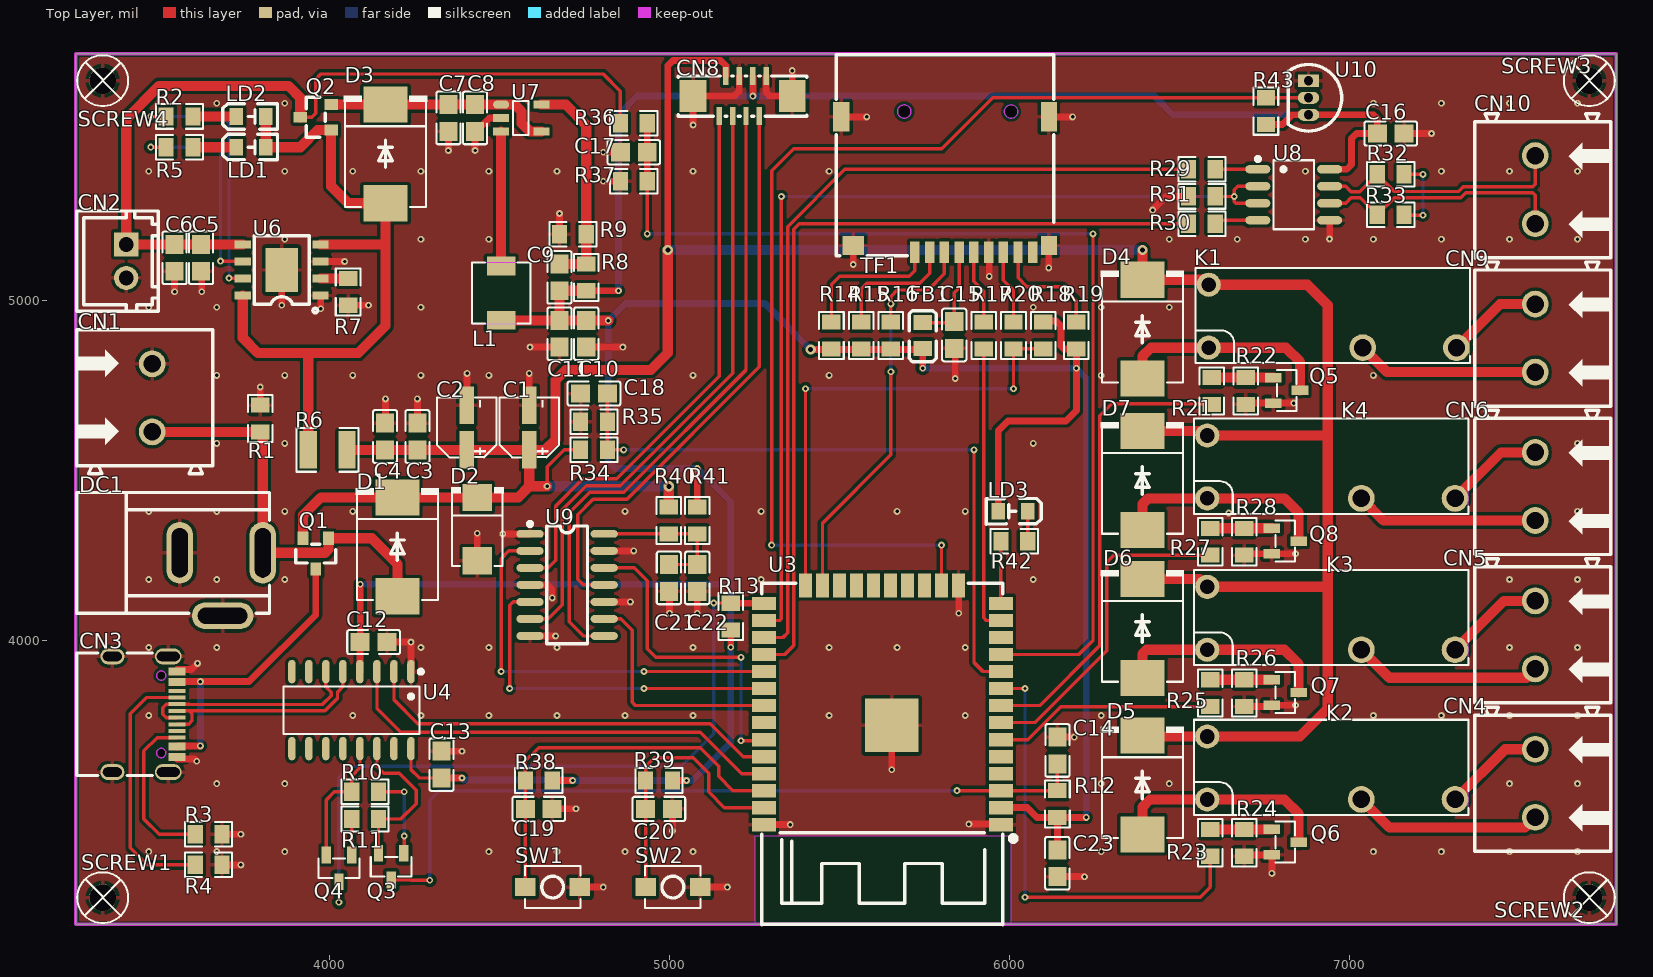
[diagram p0: Top Layer view]
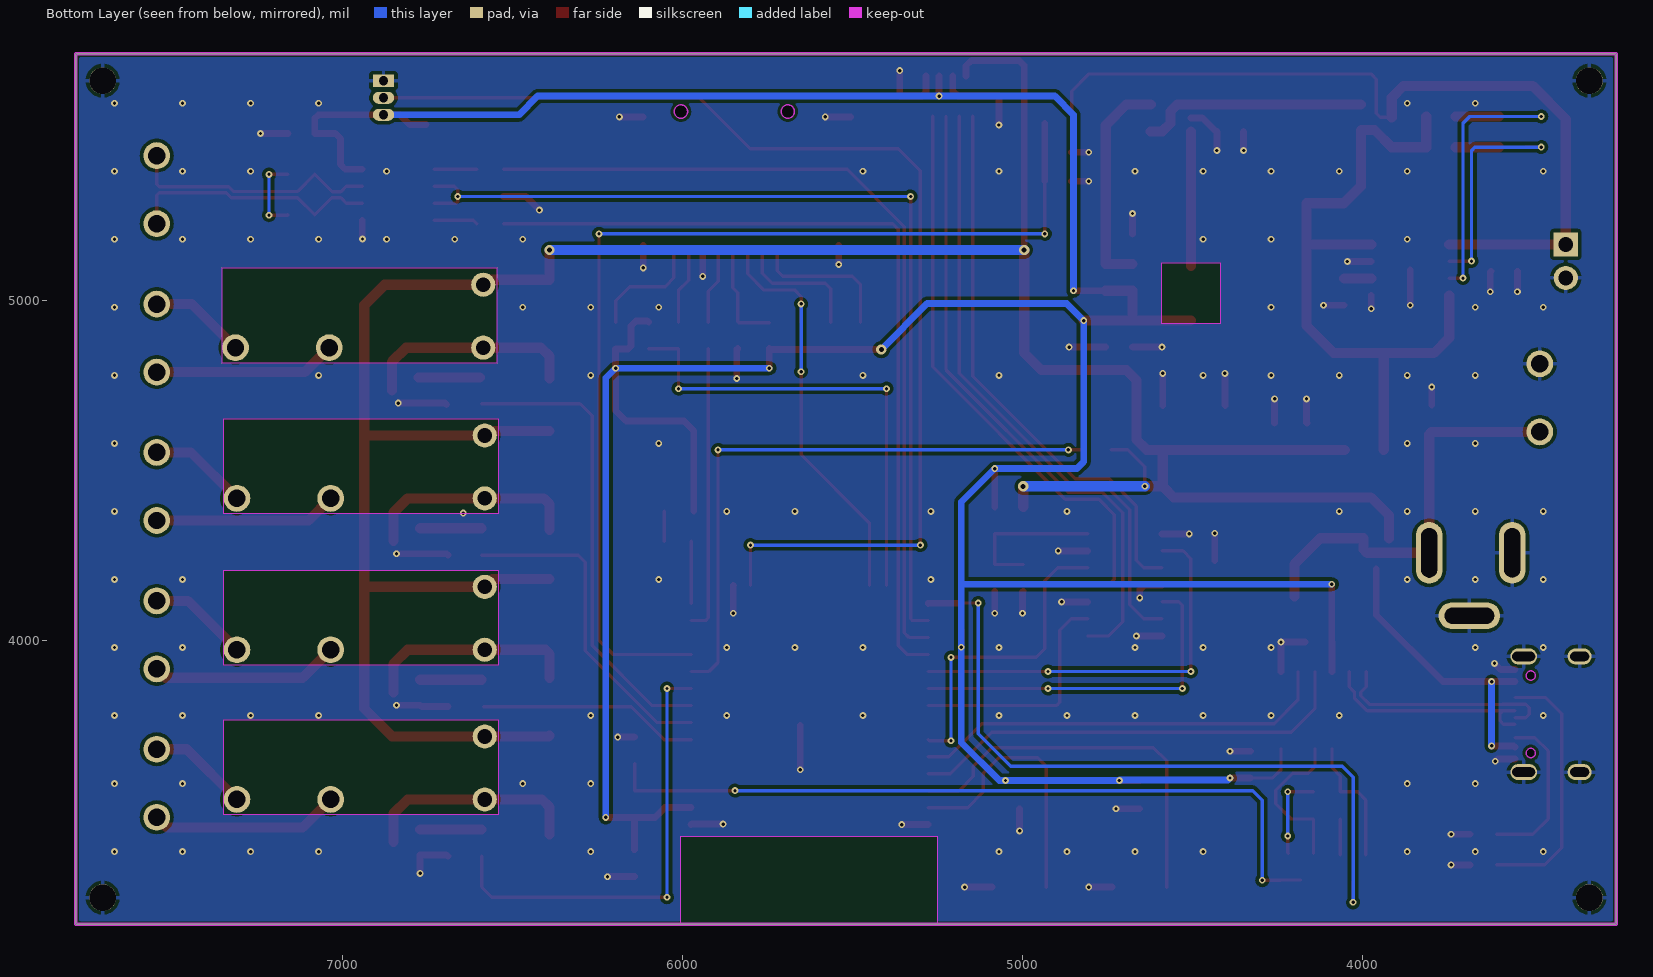
[diagram p1: Bottom Layer view, seen from below]
# Altium PCB MISC49869.pcbdoc
Units mil, origin at the board's own origin, x right, y up, seen from the top; angles counter-clockwise.
Board outline 4527.56 x 2559.06 mil, 2 copper layers (Top Layer, Bottom Layer), stack 62.206 mil thick; 114 components, 80 nets, 367 pads, 217 vias.

## Layer stack, top to bottom
Top Solder Mask Layer: solder mask 0.394, Dk 3.3
Top Layer: signal copper 1.379
Dielectric1: surface 59.449, FR4, Dk 4.5
Bottom Layer: signal copper 1.378
Bottom Solder Mask Layer: solder mask 0.394, Dk 3.3

## Board outline
3255,3165 7782.56,3165 7782.56,5724.06 3255,5724.06

## Design rules (kind name [scope] priority, off if disabled: settings)
BoardOutlineClearance copperThickness2oz_1 [All] p2 off: genericclearance=7.99 ignorepadtopadclearanceinfootprint=FALSE except(0: Arc-SplitContinuation Track-SplitContinuation SMDPad-SplitContinuation THPad-SplitContinuation Via-SplitContinuation Fill-SplitContinuation Region-SplitContinuation Poly-SplitContinuation Text-SplitContinuation Hole-SplitContinuation; 5.98: Arc-CutoutEdge Track-CutoutEdge SMDPad-CutoutEdge THPad-CutoutEdge Via-CutoutEdge Text-CutoutEdge; 6.89: Hole-OutlineEdge Hole-CutoutEdge; 10: Poly-OutlineEdge Poly-CutoutEdge; 11.81: Arc-OutlineEdge Track-OutlineEdge SMDPad-OutlineEdge THPad-OutlineEdge Via-OutlineEdge Fill-OutlineEdge Region-OutlineEdge Text-OutlineEdge Fill-CutoutEdge Region-CutoutEdge)
BoardOutlineClearance Plane_innerPlane_1 [All] p4 off: genericclearance=8 ignorepadtopadclearanceinfootprint=FALSE except(0: Arc-SplitContinuation Track-SplitContinuation SMDPad-SplitContinuation THPad-SplitContinuation Via-SplitContinuation Fill-SplitContinuation Region-SplitContinuation Poly-SplitContinuation Text-SplitContinuation Hole-SplitContinuation; 7: SMDPad-CutoutEdge THPad-CutoutEdge; 8: Arc-OutlineEdge Track-OutlineEdge SMDPad-OutlineEdge THPad-OutlineEdge Via-OutlineEdge Fill-OutlineEdge Region-OutlineEdge Text-OutlineEdge Hole-OutlineEdge Arc-CutoutEdge Track-CutoutEdge Via-CutoutEdge Fill-CutoutEdge Region-CutoutEdge Text-CutoutEdge Hole-CutoutEdge; 10: Poly-OutlineEdge Poly-CutoutEdge)
BoardOutlineClearance Copper_copperRegion_1 [All] p6 off: genericclearance=8 ignorepadtopadclearanceinfootprint=FALSE except(0: Arc-SplitContinuation Track-SplitContinuation SMDPad-SplitContinuation THPad-SplitContinuation Via-SplitContinuation Fill-SplitContinuation Region-SplitContinuation Poly-SplitContinuation Text-SplitContinuation Hole-SplitContinuation; 7: SMDPad-CutoutEdge THPad-CutoutEdge; 8: Arc-OutlineEdge Track-OutlineEdge SMDPad-OutlineEdge THPad-OutlineEdge Via-OutlineEdge Fill-OutlineEdge Region-OutlineEdge Text-OutlineEdge Hole-OutlineEdge Arc-CutoutEdge Track-CutoutEdge Via-CutoutEdge Fill-CutoutEdge Region-CutoutEdge Text-CutoutEdge Hole-CutoutEdge; 10: Poly-OutlineEdge Poly-CutoutEdge)
BoardOutlineClearance copperThickness1oz_1 [All] p8: genericclearance=8 ignorepadtopadclearanceinfootprint=FALSE except(0: Arc-SplitContinuation Track-SplitContinuation SMDPad-SplitContinuation THPad-SplitContinuation Via-SplitContinuation Fill-SplitContinuation Region-SplitContinuation Poly-SplitContinuation Text-SplitContinuation Hole-SplitContinuation; 7: SMDPad-CutoutEdge THPad-CutoutEdge; 8: Arc-OutlineEdge Track-OutlineEdge SMDPad-OutlineEdge THPad-OutlineEdge Via-OutlineEdge Fill-OutlineEdge Region-OutlineEdge Text-OutlineEdge Hole-OutlineEdge Arc-CutoutEdge Track-CutoutEdge Via-CutoutEdge Fill-CutoutEdge Region-CutoutEdge Text-CutoutEdge Hole-CutoutEdge; 10: Poly-OutlineEdge Poly-CutoutEdge)
Clearance copperThickness2oz [All] p1 off: gap=7.99 ignorepadtopadclearanceinfootprint=FALSE except(5.98: SMDPad-Track SMDPad-SMDPad THPad-Track SMDPad-THPad THPad-THPad Track-Via SMDPad-Via THPad-Via Via-Via Fill-SMDPad Region-SMDPad Fill-THPad Region-THPad Fill-Via Region-Via Fill-Fill Fill-Region Region-Region Arc-Track Arc-SMDPad Arc-THPad Arc-Via Fill-Arc Region-Arc Arc-Arc Text-Track SMDPad-Text Text-THPad Text-Via Fill-Text Region-Text Arc-Text Text-Text; 6.89: Hole-Track Hole-SMDPad Hole-THPad Hole-Via Fill-Hole Region-Hole Hole-Arc Hole-Text; 10: Poly-Track Poly-SMDPad Poly-THPad Poly-Via Poly-Fill Poly-Region Poly-Poly Poly-Arc Poly-Text Poly-Hole; 11.81: Fill-Track Region-Track)
Clearance Plane_innerPlane [All] p3 off: gap=8 ignorepadtopadclearanceinfootprint=FALSE except(7: SMDPad-SMDPad SMDPad-THPad THPad-THPad; 10: Poly-Track Poly-SMDPad Poly-THPad Poly-Via Poly-Fill Poly-Region Poly-Poly Poly-Arc Poly-Text Poly-Hole)
Clearance Copper_copperRegion [All] p5 off: gap=8 ignorepadtopadclearanceinfootprint=FALSE except(7: SMDPad-SMDPad SMDPad-THPad THPad-THPad; 10: Poly-Track Poly-SMDPad Poly-THPad Poly-Via Poly-Fill Poly-Region Poly-Poly Poly-Arc Poly-Text Poly-Hole)
Clearance copperThickness1oz [All] p7: gap=8 ignorepadtopadclearanceinfootprint=FALSE except(7: SMDPad-SMDPad SMDPad-THPad THPad-THPad; 10: Poly-Track Poly-SMDPad Poly-THPad Poly-Via Poly-Fill Poly-Region Poly-Poly Poly-Arc Poly-Text Poly-Hole)
DiffPairsRouting differentialPair [All] p1: maxlimit=8 minlimit=8 mostfreqgap=8 toplayer_minwidth=10 toplayer_prefwidth=10 toplayer_maxwidth=100 toplayer_mingap=8 toplayer_prefgap=8 toplayer_maxgap=8 bottomlayer_minwidth=10 bottomlayer_prefwidth=10 bottomlayer_maxwidth=100 bottomlayer_mingap=8 bottomlayer_prefgap=8 bottomlayer_maxgap=8 maxuncoupledlength=8
HoleToHoleClearance otherClearance [All] p1: gap=11.81 allowstackedmicrovias=TRUE
Length netLength [All] p1: minlimit=0 maxlimit=0
PasteMaskExpansion pasteMaskExpansion [All] p1: expansion=0
PlaneConnect innerPlane [All] p1: planeconnectstyle=Relief reliefexpansion=20 reliefentries=4 reliefconductorwidth=10 reliefairgap=10
PolygonConnect copperRegion [All] p1: connectstyle=Relief reliefconductorwidth=10 reliefentries=4 polygonreliefangle="90 Angle" airgapwidth=10 via.connectstyle=Relief via.reliefconductorwidth=10 via.reliefentries=4 via.polygonreliefangle="90 Angle" via.airgapwidth=10
RoutingVias viaSize [All] p1: holewidth=10 width=20 viastyle="Through Hole" minholewidth=10 minwidth=20 maxholewidth=248.03 maxwidth=393.7
SolderMaskExpansion solderMaskExpansion [IsVia] p1: expansion=-1000 istentingtop=TRUE
SolderMaskExpansion solderMaskExpansion [All] p2: expansion=2.01 istentingtop=FALSE
Width copperThickness2oz_2 [All] p1 off: maxlimit=100 minlimit=8 preferedwidth=10
Width copperThickness1oz_2 [All] p2: maxlimit=100 minlimit=8 preferedwidth=8

## Components (designator, comment, footprint, x,y, rotation, side; value= is the part's Value field where it differs from the comment)
C1 "47uF" C_Ele_SMD_4x5.5mm 4587.93,4620.75 r90 top
C2 "47uF" C_Ele_SMD_4x5.5mm 4403.8,4620.75 r90 top
C3 "100nF" C0805 4258.8,4599.37 r270 top
C4 "10nF" C0805 4163.8,4599.37 r270 top
C5 "10uF" C0805 3622.97,5124.54 r90 top
C6 "10nF" C0805 3545,5124.54 r90 top
C7 "10uF" C0805 4349.92,5535.76 r90 top
C8 "10uF" C0805 4428.44,5535.76 r90 top
C9 "NF" C0805 4676.48,5067.13 r90 top
C10 "22uF" C0805 4755.22,4901.43 r90 top
C11 "22uF" C0805 4676.48,4901.43 r90 top
C12 "100nF" C0805 4130,3995 r0 top
C13 "100nF" C0805 4330,3635 r270 top
C14 "1uF" C0805 6140.35,3676.45 r90 top
C15 "10uF" C0805 5836.91,4897.76 r270 top
C16 "100nF" C0805 7120,5490 r0 top
C17 "100nF" C0805 4895,5435 r180 top
C18 "100nF" C0805 4777.97,4725.53 r180 top
C19 "100nF" C0805 4615.7,3504.84 r180 top
C20 "100nF" C0805 4968.94,3504.84 r180 top
C21 "100nF" C0805 4997.99,4183.61 r90 top
C22 "10nF" C0805 5081.52,4183.61 r90 top
C23 "100nF" C0805 6140,3345 r270 top
CN1 "" CONN-TH_2P-P5.00_WJ500V-5.08-2P 3479.21,4712.95 r90 top
CN2 "" CONN-TH_2P-P2.50_HX25003-2A 3402.83,5114.7 r270 top
CN3 "" USB_TYPE-C-16P 3457.17,3787.83 r270 top
CN4 "" CONN-TH_2P-P5.00_WJ500V-5.08-2P 7545,3580 r270 top locked
CN5 "" CONN-TH_2P-P5.00_WJ500V-5.08-2P 7545,4016.2 r270 top locked
CN6 "" CONN-TH_2P-P5.00_WJ500V-5.08-2P 7545,4452.5 r270 top locked
CN8 "" FPC-SMD_8P-P0.50_AFC11-S08ICC-00 5215,5600 r0 top
CN9 "" CONN-TH_2P-P5.00_WJ500V-5.08-2P 7545,4888.7 r270 top locked
CN10 "" CONN-TH_2P-P5.00_WJ500V-5.08-2P 7545,5325 r270 top locked
D1 "" SMC_L6.9-W5.9-LS7.9-RD 4200,4275 r270 top
D2 "" SMB_L4.6-W3.6-LS5.3-RD 4435,4327.19 r270 top
D3 "" SMC_L6.9-W5.9-LS7.9-RD 4165,5430 r270 top
D4 "" SMC_L6.9-W5.9-LS7.9-RD 6390,4915 r270 top
D5 "" SMC_L6.9-W5.9-LS7.9-RD 6390,3575 r270 top
D6 "" SMC_L6.9-W5.9-LS7.9-RD 6390,4035 r270 top
D7 "" SMC_L6.9-W5.9-LS7.9-RD 6390,4470 r270 top
DC1 "" DC-005_2.5 3677.36,4245 r180 top
FB1 "10uH" L0805 5744.14,4896.17 r90 top
K1 "" RELAY-TH_G5NB-1A-E-DCXX 6949.3,4953.03 r0 top
K2 "" RELAY-TH_G5NB-1A-E-DCXX 6945,3625 r0 top
K3 "" RELAY-TH_G5NB-1A-E-DCXX 6945,4065 r0 top
K4 "" RELAY-TH_G5NB-1A-E-DCXX 6945,4510 r0 top
L1 "2.2uH" IND-SMD_L4.4-W4.2 4505,5020.64 r90 top
LD1 "" LED_0805 3771.66,5449.74 r0 top
LD2 "" LED_0805 3771.66,5539.92 r0 top
LD3 "" LED_0805 6007.53,4380 r180 top
Q1 "" SOT-23_L2.9-W1.3-P1.90-LS2.4-BR 3960,4255 r90 top
Q2 "" SOT-23_L2.9-W1.3-P1.90-LS2.4-BR 3960,5537.73 r0 top
Q3 "" SOT-23-3_L2.9-W1.3-P1.90-LS2.4-BR 4181.77,3335 r90 top
Q4 "" SOT-23-3_L2.9-W1.3-P1.90-LS2.4-BR 4028.23,3330 r90 top
Q5 "" SOT-23-3_L2.9-W1.3-P1.90-LS2.4-BR 6814.3,4735 r180 top
Q6 "" SOT-23-3_L2.9-W1.3-P1.90-LS2.4-BR 6810,3406.97 r180 top
Q7 "" SOT-23-3_L2.9-W1.3-P1.90-LS2.4-BR 6810,3846.97 r180 top
Q8 "" SOT-23-3_L2.9-W1.3-P1.90-LS2.4-BR 6810,4291.97 r180 top
R1 "10K" R0805 3797.04,4652.32 r270 top
R2 "1.5K" R0805 3559.69,5540.12 r0 top
R3 "5.1K" R0805 3645,3430 r180 top
R4 "5.1K" R0805 3645,3340 r180 top
R5 "1.5K" R0805 3559.69,5449.94 r0 top
R6 "100mΩ" R1210 3995,4560 r180 top
R7 "1.5K" R0805 4055,5024.54 r270 top
R8 "180K" R0805 4755.22,5067.13 r270 top
R9 "40K" R0805 4715.85,5194.4 r0 top
R10 "1K" R0805 4105,3555 r180 top
R11 "1K" R0805 4105,3475 r0 top
R12 "10K" R0805 6140.35,3519.14 r270 top
R13 "10K" R0805 5180,4070 r270 top
R14 "2.2K" R0805 5476.02,4896.17 r270 top
R15 "2.2K" R0805 5563.43,4896.17 r270 top
R16 "10K" R0805 5650.84,4896.17 r270 top
R17 "10R" R0805 5923.79,4896.17 r270 top
R18 "2.2K" R0805 6098.61,4896.17 r90 top
R19 "2.2K" R0805 6196.02,4896.17 r270 top
R20 "220R" R0805 6011.2,4896.17 r270 top
R21 "4.7K" R0805 6594.3,4733.03 r270 top
R22 "4.7K" R0805 6693.38,4733.03 r90 top
R23 "4.7K" R0805 6590,3405 r270 top
R24 "4.7K" R0805 6689.08,3405 r90 top
R25 "4.7K" R0805 6590,3845 r270 top
R26 "4.7K" R0805 6689.08,3845 r90 top
R27 "4.7K" R0805 6590,4290 r270 top
R28 "4.7K" R0805 6689.08,4290 r90 top
R29 "300R" R0805 6565,5385 r180 top
R30 "300R" R0805 6565,5225 r180 top
R31 "10K" R0805 6565,5305 r180 top
R32 "120R" R0805 7120,5370 r0 top
R33 "0R" R0805 7120,5250.89 r0 top
R34 "100K" R0805 4777.97,4560 r0 top
R35 "100K" R0805 4777.97,4643.03 r180 top
R36 "100K" R0805 4895,5520 r180 top
R37 "100K" R0805 4895,5350 r0 top
R38 "10K" R0805 4615.7,3588.13 r0 top
R39 "10K" R0805 4968.94,3588.13 r0 top
R40 "0R" R0805 4997.99,4352.42 r90 top
R41 "0R" R0805 5081.52,4352.42 r90 top
R42 "1.5K" R0805 6013.44,4291.81 r180 top
R43 "4.7K" R0805 6753.35,5555.7 r270 top
SCREW1 "" M2螺丝 3333.7,3243.7 r0 top locked
SCREW2 "" M2螺丝 7703.8,3243.7 r0 top locked
SCREW3 "" M2螺丝 7703.8,5645.3 r0 top locked
SCREW4 "" M2螺丝 3333.7,5645.3 r0 top locked
SW1 "" Key_SMD_3x4x2 4656.45,3274.84 r0 top
SW2 "" Key_SMD_3x4x2 5009.69,3274.84 r0 top
TF1 "" TF-SMD_TF-CARD-H1.8 5810,5340 r180 top
U3 "" WIFIM-SMD_ESP-WROOM-32 5625.62,3810.1 r180 top
U4 "" SOP-16_L10.0-W3.9-P1.27-LS6.0-BL 4065,3795 r180 top
U6 "" ESOP-8_L4.9-W3.9-P1.27-LS6.0-BL-EP 3860.04,5088.91 r90 top
U7 "" SOT_XDC 4505,5575.13 r0 top
U8 "" SOP-8_L4.9-W3.9-P1.27-LS6.0-BL 6835,5310 r270 top
U9 "" SOIC-14_L8.6-W3.8-P1.27-LS6.0-BL 4698.91,4163.05 r270 top
U10 "" TO-92-3_L4.9-W3.7-P1.27-L 6878.35,5595.07 r270 top

## Footprints (in the part's own frame and the unit in brackets; to place one, negate y for a bottom-side part, rotate by r counter-clockwise, add the part's x,y. Pads: shape width x height; smd on the part's side, far side on the other; paste and mask are expansions set on the pad)
C0805 [mm]
  rect 1.41x1.35 smd paste-100 mask+0.051: 1(-1,0) 2(1,0)
  silkscreen extent -1.96,-0.9 1.96,0.9
C_Ele_SMD_4x5.5mm [mm]
  rect 2.8x1.1 smd paste+0 mask+0.051: 1(-1.543,0) 2(1.778,0)
  silkscreen extent -2.1,-2.23 2.35,2.23
CONN-TH_2P-P2.50_HX25003-2A [mm]
  rect 1.8x1.8 hole 1.1 paste+0 mask+0.05: 1(-1.25,0)
  round 1.8 hole 1.1 paste+0 mask+0.05: 2(1.25,0)
  silkscreen extent -3.75,-3.7 3.75,2.41
CONN-TH_2P-P5.00_WJ500V-5.08-2P [mm]
  round 2 hole 1.3: 1(-2.54,0) 2(2.54,0)
  silkscreen extent -5.68,-4.52 5.08,5.64
DC-005_2.5 [mm]
  oval 2x4.6 hole 1.2 slot 3.7 at 90 deg paste+0 mask+0.051: 1(-3.227,-0.318) 2(2.973,-0.318)
  oval 4.6x2 hole 1.2 slot 3.7 at 0 deg paste+0 mask+0.051: 3(-0.227,4.382)
  silkscreen extent -3.73,-4.82 10.67,4.18
ESOP-8_L4.9-W3.9-P1.27-LS6.0-BL-EP [mm]
  rect 0.6x1.2 smd: 1(-1.905,-2.908) 2(-0.635,-2.908) 3(0.635,-2.908) 4(1.905,-2.908) 5(1.905,2.908) 6(0.635,2.908) 7(-0.635,2.908) 8(-1.905,2.908)
  rect 3.3x2.4 smd: 9(0,0)
  silkscreen extent -3.2,-2.67 2.55,2.05
FPC-SMD_8P-P0.50_AFC11-S08ICC-00 [mm]
  rect 0.4x1.35 smd: 1(-1.75,-1.5) 2(-1.25,1.5) 3(-0.75,-1.5) 4(-0.25,1.5) 5(0.25,-1.5) 6(0.75,1.5) 7(1.25,-1.5) 8(1.75,1.5)
  rect 2x2.4 smd: 9(3.7,0) 10(-3.7,0)
  silkscreen extent -4.81,-1.5 4.8,1.5
IND-SMD_L4.4-W4.2 [mm]
  rect 1.4x2.12 smd: 1(2.028,0) 2(-2.028,0)
  silkscreen extent -2.28,-2.18 2.28,2.18
Key_SMD_3x4x2 [mm]
  rect 1.53x1.36 smd paste+0 mask+0.051: 1(-2.035,0) 2(2.035,0)
  silkscreen extent -2.08,-1.58 2.08,1.58
L0805 [mil]
  rect 44.59x54.21 smd paste-3937.01 mask+2: 1(-38.04,0) 2(38.04,0)
  silkscreen extent -77,-40 73,40
LED_0805 [mm]
  rect 1x1.25 smd paste+0 mask+0.051: 1(-1.15,0.005) 2(1.05,0.005)
  silkscreen extent -2.15,-0.94 1.93,0.97
M2螺丝 [mm]
  round 2 hole 2: 1(0,0)
  silkscreen extent -1.9,-1.9 1.9,1.9
R0805 [mm]
  rect 1.133x1.377 smd paste-100 mask+0.051: 1(-1,0) 2(1,0)
  silkscreen extent -1.76,-0.92 1.76,0.92
R1210 [mil]
  rect 50.49x110.55 smd paste-3937.01 mask+2: 1(-56.74,0) 2(56.74,0)
  silkscreen extent -91,-64 91,64
RELAY-TH_G5NB-1A-E-DCXX [mm]
  round 1.8 hole 1.1: 1(-9.25,-2.35) 4(-9.25,2.35)
  round 2 hole 1.3: 2(2.25,-2.35) 3(9.25,-2.35)
  silkscreen extent -10.25,-3.5 10.25,3.6
SMB_L4.6-W3.6-LS5.3-RD [mil]
  rect 80.61x86.31 smd: 1(-92.94,0) 2(92.94,0)
  silkscreen extent -123,-77 108,77
SMC_L6.9-W5.9-LS7.9-RD [mm]
  rect 2.7x3.3 smd: 1(-3.686,0) 2(3.686,0)
  silkscreen extent -4.36,-3.1 3.98,3.1
SOIC-14_L8.6-W3.8-P1.27-LS6.0-BL [mil]
  oval 22.6x80.24 smd: 1(-150,-109.02) 2(-100,-109.02) 3(-50,-109.02) 4(0,-109.02) 5(50,-109.02) 6(100,-109.02) 7(150,-109.02) 8(150,109.02) 9(100,109.02) 10(50,109.02) 11(0,109.02) 12(-50,109.02) 13(-100,109.02) 14(-150,109.02)
  silkscreen extent -185,-115 173,60
SOP-8_L4.9-W3.9-P1.27-LS6.0-BL [mm]
  oval 0.63x1.865 smd: 1(-1.905,-2.682) 2(-0.635,-2.682) 3(0.635,-2.682) 4(1.905,-2.682) 5(1.905,2.682) 6(0.635,2.682) 7(-0.635,2.682) 8(-1.905,2.682)
  silkscreen extent -2.82,-2.83 2.58,1.52
SOP-16_L10.0-W3.9-P1.27-LS6.0-BL [mm]
  oval 0.56x1.745 smd: 1(-4.445,-2.872) 2(-3.175,-2.872) 3(-1.905,-2.872) 4(-0.635,-2.872) 5(0.635,-2.872) 6(1.905,-2.872) 7(3.175,-2.872) 8(4.445,-2.872) 9(4.445,2.872) 10(3.175,2.872) 11(1.905,2.872) 12(0.635,2.872) 13(-0.635,2.872) 14(-1.905,2.872) 15(-3.175,2.872) 16(-4.445,2.872)
  silkscreen extent -5.33,-3.02 5.08,1.77
SOT-23-3_L2.9-W1.3-P1.90-LS2.4-BR [mm]
  rect 1.25x0.7 smd: 1(1,-0.95) 2(1,0.95) 3(-1,0)
  silkscreen extent -0.73,-1.53 0.73,1.53
SOT-23_L2.9-W1.3-P1.90-LS2.4-BR [mm]
  rect 1x0.8 smd: 1(1.15,-0.95) 2(1.15,0.95) 3(-1.15,0)
  silkscreen extent -0.7,-1.5 0.7,1.5
SOT_XDC [mm]
  oval 1.2x0.6 smd: 1(0,0)
  rect 1.2x0.6 smd: 2(0,-1) 3(0,-2) 4(3,-2) 5(3,0)
  silkscreen extent 0.89,-2.29 2.03,0.25
TF-SMD_TF-CARD-H1.8 [mm]
  rect 0.7x1.6 smd paste+0 mask+0.05: 1(2.25,5.05) 2(1.15,5.05) 3(0.05,5.05) 4(-1.05,5.05) 5(-2.15,5.05) 6(-3.25,5.05) 7(-4.35,5.05) 8(-5.45,5.05) 9(-6.55,5.05)
  rect 1.2x1.4 smd paste+0 mask+0.05: 10(-7.747,4.55)
  rect 1.2x2.2 smd paste+0 mask+0.05: 11(-7.75,-5.05) 12(7.75,-5.05)
  rect 1.6x1.4 smd paste+0 mask+0.05: 13(6.85,4.55)
  Board Outline Layer circle w0.003: c3.05,-5.45 r0.5
  Board Outline Layer circle w0.003: c-4.93,-5.45 r0.5
  Board Outline Layer region: 2.55,-5.45 2.6,-5.233 2.738,-5.059 2.939,-4.962 3.161,-4.962 3.362,-5.059 3.501,-5.233 3.55,-5.45 3.55,-5.45 3.501,-5.667 3.362,-5.841 3.161,-5.937 2.939,-5.937 2.738,-5.841 2.6,-5.667 2.55,-5.45
  Board Outline Layer region: 2.55,-5.45 2.56,-5.352 2.588,-5.259 2.634,-5.172 2.696,-5.096 2.772,-5.034 2.859,-4.988 2.952,-4.96 3.05,-4.95 3.148,-4.96 3.241,-4.988 3.328,-5.034 3.404,-5.096 3.466,-5.172 3.512,-5.259 3.54,-5.352 3.55,-5.45 3.54,-5.547 3.512,-5.641 3.466,-5.728 3.404,-5.804 3.328,-5.866 3.241,-5.912 3.148,-5.94 3.05,-5.95 2.952,-5.94 2.859,-5.912 2.772,-5.866 2.696,-5.804 2.634,-5.728 2.588,-5.641 2.56,-5.547
  Board Outline Layer region: -5.43,-5.45 -5.381,-5.233 -5.242,-5.059 -5.041,-4.962 -4.819,-4.962 -4.618,-5.059 -4.48,-5.233 -4.43,-5.45 -4.43,-5.45 -4.48,-5.667 -4.618,-5.841 -4.819,-5.937 -5.041,-5.937 -5.242,-5.841 -5.381,-5.667 -5.43,-5.45
  Board Outline Layer region: -5.43,-5.45 -5.421,-5.352 -5.392,-5.259 -5.346,-5.172 -5.284,-5.096 -5.208,-5.034 -5.121,-4.988 -5.028,-4.96 -4.93,-4.95 -4.833,-4.96 -4.739,-4.988 -4.652,-5.034 -4.577,-5.096 -4.514,-5.172 -4.468,-5.259 -4.44,-5.352 -4.43,-5.45 -4.44,-5.547 -4.468,-5.641 -4.514,-5.728 -4.577,-5.804 -4.652,-5.866 -4.739,-5.912 -4.833,-5.94 -4.93,-5.95 -5.028,-5.94 -5.121,-5.912 -5.208,-5.866 -5.284,-5.804 -5.346,-5.728 -5.392,-5.641 -5.421,-5.547
  Multi-Layer board cut-out: 2.55,-5.45 2.6,-5.233 2.738,-5.059 2.939,-4.962 3.161,-4.962 3.362,-5.059 3.501,-5.233 3.55,-5.45 3.55,-5.45 3.501,-5.667 3.362,-5.841 3.161,-5.937 2.939,-5.937 2.738,-5.841 2.6,-5.667 2.55,-5.45
  Multi-Layer board cut-out: -5.43,-5.45 -5.381,-5.233 -5.242,-5.059 -5.041,-4.962 -4.819,-4.962 -4.618,-5.059 -4.48,-5.233 -4.43,-5.45 -4.43,-5.45 -4.48,-5.667 -4.618,-5.841 -4.819,-5.937 -5.041,-5.937 -5.242,-5.841 -5.381,-5.667 -5.43,-5.45
  silkscreen extent -8.13,-9.68 8.13,5.3
TO-92-3_L4.9-W3.7-P1.27-L [mm]
  rect 0.9x1.6 hole 0.7 paste+0 mask+0.051: 1(-1.27,0)
  oval 0.9x1.6 hole 0.7 paste+0 mask+0.051: 2(0,0) 3(1.27,0)
  silkscreen extent -2.48,-1.5 2.48,2.48
USB_TYPE-C-16P [mm]
  oval 1.2x2 hole 0.7 slot 1.7 at 90 deg paste+0 mask+0.051: 1(-4.193,1.765) 2(4.447,1.765)
  oval 1.2x1.8 hole 0.7 slot 1.4 at 90 deg paste+0 mask+0.051: 3(-4.193,-2.415) 4(4.447,-2.415)
  rect 0.3x1.3 smd paste-100 mask+0.05: A1(-3.223,2.415) A4(-2.423,2.415) A5(-1.123,2.415) A6(-0.123,2.415) A7(0.377,2.415) A8(1.377,2.415) A9(2.677,2.415) A12(3.477,2.415) B1(3.177,2.415) B4(2.377,2.415) B5(1.877,2.415) B6(0.877,2.415) B7(-0.623,2.415) B8(-1.623,2.415) B9(-2.123,2.415) B12(-2.923,2.415)
  Board Outline Layer circle w0.003: c-2.763,1.235 r0.35
  Board Outline Layer circle w0.003: c3.017,1.235 r0.35
  Board Outline Layer region: -2.763,1.585 -2.611,1.55 -2.489,1.453 -2.422,1.313 -2.422,1.157 -2.489,1.017 -2.611,0.92 -2.763,0.885 -2.763,0.885 -2.915,0.92 -3.037,1.017 -3.104,1.157 -3.104,1.313 -3.037,1.453 -2.915,1.55 -2.763,1.585
  Board Outline Layer region: -2.763,1.585 -2.685,1.576 -2.611,1.55 -2.545,1.509 -2.489,1.453 -2.448,1.387 -2.422,1.313 -2.413,1.235 -2.422,1.157 -2.448,1.083 -2.489,1.017 -2.545,0.961 -2.611,0.92 -2.685,0.894 -2.763,0.885 -2.841,0.894 -2.915,0.92 -2.981,0.961 -3.037,1.017 -3.078,1.083 -3.104,1.157 -3.113,1.235 -3.104,1.313 -3.078,1.387 -3.037,1.453 -2.981,1.509 -2.915,1.55 -2.841,1.576
  Board Outline Layer region: 3.017,1.585 3.169,1.55 3.291,1.453 3.358,1.313 3.358,1.157 3.291,1.017 3.169,0.92 3.017,0.885 3.017,0.885 2.865,0.92 2.743,1.017 2.676,1.157 2.676,1.313 2.743,1.453 2.865,1.55 3.017,1.585
  Board Outline Layer region: 3.017,1.585 3.095,1.576 3.169,1.55 3.235,1.509 3.291,1.453 3.332,1.387 3.358,1.313 3.367,1.235 3.358,1.157 3.332,1.083 3.291,1.017 3.235,0.961 3.169,0.92 3.095,0.894 3.017,0.885 2.939,0.894 2.865,0.92 2.799,0.961 2.743,1.017 2.702,1.083 2.676,1.157 2.667,1.235 2.676,1.313 2.702,1.387 2.743,1.453 2.799,1.509 2.865,1.55 2.939,1.576
  Multi-Layer board cut-out: -2.763,1.585 -2.611,1.55 -2.489,1.453 -2.422,1.313 -2.422,1.157 -2.489,1.017 -2.611,0.92 -2.763,0.885 -2.763,0.885 -2.915,0.92 -3.037,1.017 -3.104,1.157 -3.104,1.313 -3.037,1.453 -2.915,1.55 -2.763,1.585
  Multi-Layer board cut-out: 3.017,1.585 3.169,1.55 3.291,1.453 3.358,1.313 3.358,1.157 3.291,1.017 3.169,0.92 3.017,0.885 3.017,0.885 2.865,0.92 2.743,1.017 2.676,1.157 2.676,1.313 2.743,1.453 2.865,1.55 3.017,1.585
  silkscreen extent -4.45,-5.08 4.7,0.57
WIFIM-SMD_ESP-WROOM-32 [mm]
  rect 1.8x1.001 smd: 1(-8.851,8.93) 2(-8.851,7.66) 3(-8.851,6.39) 4(-8.851,5.12) 5(-8.851,3.85) 6(-8.851,2.58) 7(-8.851,1.31) 8(-8.851,0.04) 9(-8.851,-1.23) 10(-8.851,-2.5) 11(-8.851,-3.77) 12(-8.851,-5.04) 13(-8.851,-6.31) 14(-8.851,-7.58) 25(8.851,-7.58) 26(8.851,-6.31) 27(8.851,-5.04) 28(8.851,-3.77) 29(8.851,-2.5) 30(8.851,-1.23) 31(8.851,0.04) 32(8.851,1.31) 33(8.851,2.58) 34(8.851,3.85) 35(8.851,5.12) 36(8.851,6.39) 37(8.851,7.66) 38(8.851,8.93)
  rect 1.001x1.8 smd: 15(-5.69,-8.93) 16(-4.42,-8.93) 17(-3.15,-8.93) 18(-1.88,-8.93) 19(-0.61,-8.93) 20(0.66,-8.93) 21(1.93,-8.93) 22(3.2,-8.93) 23(4.47,-8.93) 24(5.74,-8.93)
  rect 4x4 smd: 39(-0.7,1.52)
  silkscreen extent -9.97,-9.08 8.99,16.42

## Free pads (board coordinates)
  rect 54.21x44.59 smd paste-3937.01 mask+2: 1(6590,3884.37) 1(6590,4329.37) 1(6594.3,4772.4) 2(6689.08,3884.37) 2(6689.08,4329.37) 2(6693.38,4772.4)
  rect 49.21x27.56 smd: 1(6770.63,3884.37) 1(6770.63,4329.37) 1(6774.93,4772.4)

## Via types
v1: diameter 20, hole 10, Top Layer to Bottom Layer, 213 vias
v2: diameter 30, hole 15, Top Layer to Bottom Layer, 4 vias

## Nets (pads, with @x,y where several pads share a name; then routed paths per layer and width w, separated by ;. In a path a pad name is that pad's centre, name@x,y a point inside that pad or via, vN(x,y) a via of type N, cw(c..) or ccw(c..) an arc to the next point about the centre after c; other vN are vias at no path point)
$1N2320: CN3.B5 R3.2 | length 482.6
  Top Layer w10: CN3.B5 3493.93,3713.93 3455,3675 3455,3475 3500,3430 R3.2
$1N2381: CN3.A5 R4.2 | length 763.1
  Top Layer w10: CN3.A5 3462.04,3832.04 3415,3785 3415,3390 3465,3340 R4.2
$1N5837: Q3.2 R11.2 U4.14 | length 465.8
  Top Layer w10: U4.14 4140,3630 4160,3610 4205,3610 4255,3560 4255,3520 4210,3475 R11.2 Q3.2
$1N5841: Q4.2 R10.2 U4.13 | length 383.3
  Top Layer w10: Q4.2 3990.83,3530.83 4015,3555 R10.2 4065.63,3600.63 4090,3625 U4.13
$1N5844: Q4.1 R11.1 | length 105.6
  Top Layer w10: Q4.1 R11.1
$1N5846: Q3.1 R10.1 | length 256.6
  Top Layer w10: R10.1 v1(4220,3555) ; Q3.1 4220,3375.2 v1(4220,3425)
  Bottom Layer w10: v1(4220,3425) v1(4220,3555)
$1N6425: R14.1 TF1.1 | length 427.4
  Top Layer w10: R14.1 5476.02,5046.02 5500,5070 5705,5070 5721.42,5086.42 TF1.1
$1N6456: R15.1 TF1.2 | length 379.8
  Top Layer w10: R15.1 5563.43,5033.43 5580,5050 5735,5050 5764.73,5079.73 TF1.2
$1N6566: C15.1 FB1.2 TF1.4 | length 304
  Top Layer w10: FB1.2 5834,4934.21 C15.1 5836.91,5021.91 5851.34,5036.34 TF1.4
$1N6650: R17.1 TF1.5 | length 217.7
  Top Layer w10: TF1.5 5894.65,5055.35 5923.79,5026.21 R17.1
$1N6781: R19.1 TF1.8 | length 338.2
  Top Layer w10: TF1.8 6024.57,5065.43 6050,5040 6155,5040 6196.02,4998.98 R19.1
$1N6830: R20.1 TF1.7 | length 218
  Top Layer w10: TF1.7 5981.26,5058.74 6011.2,5028.8 R20.1
$2N2543: LD2.1 R2.2 | length 127.3
  Top Layer w30: R2.2 LD2.1
$2N2544: LD1.1 R5.2 | length 127.3
  Top Layer w30: R5.2 LD1.1
$2N2545: R5.1 U6.6 | length 645.4
  Top Layer w10: v1(3475,5450) R5.1@3520.27,5450 ; v1(3680,5115) 3744.45,5115 U6.6
  Bottom Layer w10: v1(3475,5450) 3670,5450 3680,5440 v1(3680,5115)
$2N2546: R2.1 U6.7 | length 779.6
  Top Layer w10: v1(3475,5540) 3520.2,5540 R2.1 ; v1(3705,5065) 3744.45,5065 U6.7
  Bottom Layer w10: v1(3475,5540) 3685,5540 3705,5520 v1(3705,5065)
$2N2547: D3.2 LD1.2 LD2.2 Q2.1 R6.2 U6.4 U6.8 | length 2080.1
  Top Layer w30: U6.8 3745.54,4889.46 3790,4845 3938.26,4845 ; LD2.2 LD1.2 3914.94,5449.94 3965.33,5500.33 Q2.1 4005.28,5334.72 4055.13,5284.87 D3.2 4165,5163.91 ; R6.2 3938.26,4845 ; U6.4 4165,5163.91 ; 3938.26,4845 4085,4845 4165,4925 4165,5163.91
$2N2548: R7.1 U6.2 | length 80.5
  Top Layer w30: U6.2 R7.1
$2N8440: C9.2 R8.1 R9.2 U7.5 | length 644.1
  Top Layer w30: U7.5 4694.87,5575.13 4755.22,5514.78 R9.2 R8.1 C9.2
$2N8459: L1.1 U7.3 | length 395.9
  Top Layer w30: L1.1 U7.3
$2N8563: LD3.1 R42.1 | length 88
  Top Layer w10: R42.1 LD3.1
$3N357: D4.2 K1.1 Q5.3 | length 640.4
  Top Layer w30: D4.2 6390,4835 6415.51,4860.51 K1.1 6811.82,4860.51 6853.67,4818.66 Q5.3
$3N404: pad.1@6594.3,4772.4 pad.1@6774.93,4772.4 pad.2@6693.38,4772.4 Q5.1 R21.1 R22.2 | length 180.6
  Top Layer w30: R21.1 R22.2 Q5.1
$3N563: CN9.1 K1.3 | length 284.6
  Top Layer w30: K1.3 7441.67,4988.7 CN9.1
$3N568: CN9.2 K1.2 | length 536.9
  Top Layer w30: K1.2 7109.7,4788.7 CN9.2
$3N810: Q6.1 R23.1 R24.2 | length 180.6
  Top Layer w30: R23.1 R24.2 Q6.1
$3N823: D5.2 K2.1 Q6.3 | length 649.8
  Top Layer w30: D5.2 6390,3510 6412.48,3532.48 K2.1 6807.52,3532.48 6849.37,3490.63 Q6.3
$3N828: CN4.1 K2.3 | length 296.9
  Top Layer w30: K2.3 7456.69,3680 CN4.1
$3N831: CN4.2 K2.2 | length 558
  Top Layer w30: K2.2 7116.06,3450 7515,3450 CN4.2
$3N1300: pad.1@6590,3884.37 pad.1@6770.63,3884.37 pad.2@6689.08,3884.37 Q7.1 R25.1 R26.2 | length 180.6
  Top Layer w30: R25.1 R26.2 Q7.1
$3N1313: D6.2 K3.1 Q7.3 | length 635.7
  Top Layer w30: D6.2 6390,3960 6402.48,3972.48 K3.1 6807.52,3972.48 6849.37,3930.63 Q7.3
$3N1318: CN5.1 K3.3 | length 295.4
  Top Layer w30: K3.3 7452.9,4116.2 CN5.1
$3N1321: CN5.2 K3.2 | length 556.4
  Top Layer w30: K3.2 7116.06,3890 7518.8,3890 CN5.2
$3N1326: pad.1@6590,4329.37 pad.1@6770.63,4329.37 pad.2@6689.08,4329.37 Q8.1 R27.1 R28.2 | length 180.6
  Top Layer w30: R27.1 R28.2 Q8.1
$3N1339: D7.2 K4.1 Q8.3 | length 642.7
  Top Layer w30: D7.2 6390,4400 6407.48,4417.48 K4.1 6807.52,4417.48 6849.37,4375.63 Q8.3
$3N1344: CN6.1 K4.3 | length 291.8
  Top Layer w30: K4.3 7444.19,4552.5 CN6.1
$3N1347: CN6.2 K4.2 | length 538.3
  Top Layer w30: K4.2 7098.56,4352.5 CN6.2
$3N1624: R29.1 U8.1 | length 125
  Top Layer w10: R29.1 U8.1
$3N1654: R30.1 U8.4 | length 129.2
  Top Layer w10: R30.1 6614.37,5235 U8.4
$3N1923: R32.2 R33.2 | length 231.6
  Top Layer w10: R33.2 7160.26,5250 v1(7215,5250) ; R32.2 v1(7215,5370)
  Bottom Layer w10: v1(7215,5250) v1(7215,5370)
$3N3583: C21.2 C22.2 R40.1 R41.1 U9.14 | length 447.2
  Top Layer w10: U9.14 R40.1 R41.1 C22.2 C21.2
$3N3776: CN8.1 U9.3 | length 1648
  Top Layer w10: U9.3 4643.05,4213.05 4665,4235 4665,4395 4745,4475 4845,4475 5146.1,4776.1 CN8.1
$3N3780: CN8.3 U9.6 | length 1814
  Top Layer w10: U9.6 4643.05,4063.05 4685,4105 4685,4384.54 4755.46,4455 4855,4455 5185.47,4785.47 CN8.3
$3N3785: CN8.5 U9.8 | length 1880.2
  Top Layer w10: U9.8 4746.95,4013.05 4705,4055 4705,4375 4765.36,4435.36 4865.36,4435.36 5224.84,4794.84 CN8.5
$3N3790: CN8.7 U9.11 | length 1725.8
  Top Layer w10: U9.11 4746.95,4163.05 4730,4180 4730,4370 4775,4415 4875,4415 5264.21,4804.21 CN8.7
ADC1: C18.1 R34.2 R35.1 U3.10 | length 1958.2
  Top Layer w10: C18.1 R35.1 R34.2 v1(4865,4560) ; v1(5895,4560) 5895,3935 5921.49,3908.51 U3.10
  Bottom Layer w10: v1(4865,4560) v1(5895,4560)
ADC2: C17.1 R36.1 R37.2 U3.11 | length 3118.7
  Top Layer w10: v1(4934.37,5195) R37.2 ; U3.11 6203.51,3958.51 6245,4000 v1(6245,5195)
  Top Layer w20: R37.2 C17.1 R36.1
  Bottom Layer w10: v1(4934.37,5195) v1(6245,5195)
D+: CN3.A6 CN3.B6 U4.5 | length 653.1
  Top Layer w10: CN3.B6 3586.19,3753.3 3596.19,3763.3 3596.19,3785 3588.52,3792.67 3587.84,3792.67 ; CN3.A6 3587.84,3792.67 ; U4.5 4040,3863.74 4024,3847.74 4024,3830.28 3987.24,3793.52 3588.68,3793.52 3587.84,3792.67
D-: CN3.A7 CN3.B7 U4.6 | length 654.1
  Top Layer w10: CN3.A7 3520,3772.99 3510,3782.99 3510,3802.36 3520,3812.36 CN3.B7 3587.84,3812.36 3588.68,3811.52 3979.78,3811.52 4006,3837.74 4006,3847.74 3990,3863.74 U4.6
EN: C14.1 Q3.3 R12.1 U3.3 | length 2284.2
  Top Layer w10: Q3.3 4239.37,3295.63 4240,3295 v1(4295,3295) ; v1(5845,3558.51) U3.3 R12.1 C14.1
  Bottom Layer w10: v1(4295,3295) 4295,3530 4323.51,3558.51 v1(5845,3558.51)
GND: C1.2 C2.2 C3.1 C4.1 C5.1 C6.1 C7.1 C8.1 C10.1 C11.1 C12.2 C13.1 C14.2 C15.2 C16.2 C17.2 C18.2 C19.1 C20.1 C21.1 C22.1 C23.2 CN1.2 CN2.2 CN3.1 CN3.2 CN3.3 CN3.4 CN3.A1 CN3.A12 CN3.B1 CN3.B12 CN8.4 CN8.8 CN8.9 CN8.10 D2.2 DC1.2 DC1.3 Q5.2 Q6.2 Q7.2 Q8.2 R1.1 R3.1 R4.1 R7.2 R9.1 R22.1 R24.1 R26.1 R28.1 R31.2 R35.2 R37.1 SCREW1.1 SCREW2.1 SCREW3.1 SCREW4.1 SW1.2 SW2.2 TF1.6 TF1.10 TF1.11 TF1.12 TF1.13 U3.1 U3.15 U3.38 U3.39 U4.1 U6.1 U6.3 U6.9 U7.2 U8.5 U9.1 U9.4 U9.7 U9.10 U9.13 U10.1 | length 4968.9
  Top Layer w20: v1(3545,5025) C6.1 ; CN3.A12 3604.06,3650.94 v1(3610,3645) ; CN3.A1 3594.72,3914.72 v1(3612.5,3932.5) ; C5.1 3625,5083.14 v1(3625,5025) ; R4.1 v1(3740,3340) ; R3.1 v1(3740,3430) ; R1.1 v1(3797.04,4745) ; v1(3860.04,4985) U6.9 ; U6.1 3975,5013.45 v1(3975,4975) ; U6.3 v1(4045,5113.91) ; R7.2 v1(4115,4985.17) ; C4.1 4165,4639.94 v1(4165,4710) ; C12.2 v1(4240,3995) U4.1 ; C3.1 v1(4258.8,4710) ; C13.1 v1(4390,3674.37) ; C7.1 4350,5496.31 v1(4350,5440) ; C2.2 4405,4691.95 v1(4405,4785) ; v1(4428.44,5440) C8.1 4431.39,5496.39 4470.76,5535.76 U7.2 ; D2.2 v1(4435,4315) ; v1(4510,4313.05) U9.1 ; C1.2 v1(4587.93,4785) ; U9.7 v1(4665,4013.05) ; U9.4 4641.95,4163.05 4655,4150 v1(4655,4125) ; v1(4590,4862.06) C11.1 ; C19.1 v1(4725,3504.84) ; R9.1 v1(4676.48,5255) ; SW1.2 v1(4805,3274.84) ; C10.1 v1(4862.94,4862.06) ; v1(4805,5350) R37.1 ; v1(4805,5435) C17.2 ; U9.10 v1(4885,4113.05) ; U9.13 v1(4895,4263.05) ; C21.1 5000,4142.23 v1(5000,4080) ; v1(5008.31,3440) C20.1 ; v1(5069.33,5515) CN8.10 5190.01,5600.01 5205.16,5615.16 CN8.4 ; v1(5081.52,4080) C22.1 ; SW2.2 v1(5170,3274.84) ; U3.38 v1(5355,3458.51) ; CN8.8 5283.89,5611.11 5295,5600 CN8.9 v1(5360.67,5675) ; TF1.12 v1(5580,5538.81) ; v1(5540.32,5105) TF1.13 ; v1(5653.19,3620) U3.39 ; C15.2 5840,4855.3 v1(5840,4770) ; U3.15 5850,4161.31 v1(5850,4080) ; v1(5880,3460) 5972.58,3460 U3.1 ; TF1.6 5940,5139.15 v1(5940,5070) ; v1(6115,5095) TF1.10 ; TF1.11 v1(6185,5538.81) ; C23.2 6219.37,3305.63 v1(6220,3305) ; C14.2 v1(6190,3715.82) ; v1(6420,5265) 6460,5305 R31.2 ; R24.1 6693.02,3369.57 Q6.2 v1(6770.63,3315) ; R26.1 6766.69,3805.63 Q7.2 v1(6840,3809.57) ; R28.1 6693.02,4254.57 Q8.2 v1(6840,4254.57) ; R22.1 6697.32,4697.6 Q5.2 v1(6835,4697.6) ; v1(6940,5180) 6940.61,5180.61 U8.5 ; C16.2 v1(7240,5490)
  other v1: 3469.1,3379.1 3669.1,3379.1 3869.1,3379.1 4469.1,3379.1 4669.1,3379.1 4869.1,3379.1 5069.1,3379.1 6269.1,3379.1 7069.1,3379.1 7269.1,3379.1 7469.1,3379.1 7669.1,3379.1 3669.1,3579.1 3869.1,3579.1 6269.1,3579.1 6469.1,3579.1 7469.1,3579.1 7669.1,3579.1 3469.1,3779.1 4069.1,3779.1 4269.1,3779.1 4469.1,3779.1 4669.1,3779.1 4869.1,3779.1 5069.1,3779.1 5469.1,3779.1 5869.1,3779.1 6269.1,3779.1 7069.1,3779.1 7269.1,3779.1 7469.1,3779.1 7669.1,3779.1 3469.1,3979.1 3669.1,3979.1 4269.1,3979.1 4469.1,3979.1 4669.1,3979.1 5069.1,3979.1 5469.1,3979.1 5669.1,3979.1 5869.1,3979.1 7469.1,3979.1 7669.1,3979.1 3469.1,4179.1 3669.1,4179.1 3869.1,4179.1 5269.1,4179.1 6069.1,4179.1 7469.1,4179.1 7669.1,4179.1 6644.1,4374.1 3469.1,4379.1 3669.1,4379.1 3869.1,4379.1 4069.1,4379.1 4869.1,4379.1 5269.1,4379.1 5669.1,4379.1 5869.1,4379.1 7669.1,4379.1 3669.1,4579.1 3869.1,4579.1 6069.1,4579.1 7669.1,4579.1 3669.1,4779.1 3869.1,4779.1 4069.1,4779.1 4269.1,4779.1 4469.1,4779.1 5069.1,4779.1 5469.1,4779.1 6269.1,4779.1 7069.1,4779.1 7669.1,4779.1 3469.1,4979.1 3669.1,4979.1 4269.1,4979.1 6069.1,4979.1 6269.1,4979.1 6469.1,4979.1 7669.1,4979.1 3869.1,5179.1 4269.1,5179.1 4469.1,5179.1 6469.1,5179.1 6669.1,5179.1 6869.1,5179.1 7069.1,5179.1 7269.1,5179.1 7469.1,5179.1 7669.1,5179.1 3469.1,5379.1 3869.1,5379.1 4069.1,5379.1 4269.1,5379.1 4469.1,5379.1 4669.1,5379.1 5069.1,5379.1 5469.1,5379.1 6869.1,5379.1 7269.1,5379.1 7469.1,5379.1 7669.1,5379.1 3669.1,5579.1 3869.1,5579.1 7069.1,5579.1 7269.1,5579.1 7469.1,5579.1 7669.1,5579.1
IO0: Q4.3 R13.1 U3.25 | length 2115.9
  Top Layer w10: v1(4028.23,3230) Q4.3 ; v1(5130,4110) 5179.37,4110 R13.1
  Top Layer w20: R13.1 5276.32,4109.37 U3.25
  Bottom Layer w10: v1(4028.23,3230) 4028.23,3598.23 4060,3630 5035,3630 5130,3725 v1(5130,4110)
IO2: R18.1 R20.2 U3.24 | length 1394.1
  Top Layer w10: U3.24 v1(5399.62,4740) ; v1(6011.2,4740) R20.2 R18.1
  Bottom Layer w10: v1(5399.62,4740) v1(6011.2,4740)
IO4: R31.1 U3.26 U8.2 U8.3 | length 2861.7
  Top Layer w10: U3.26 5323.51,4058.51 5329,4064 v1(5329,5305) ; R31.1 v1(6660,5305) ; U8.3 6665,5285 6660,5290 v1(6660,5305) ; U8.2 6670,5335 6660,5325 v1(6660,5305)
  Bottom Layer w10: v1(5329,5305) v1(6660,5305)
IO5: U3.29 U9.2 | length 1198.1
  Top Layer w10: v1(4505,3908.51) 4505,4240 4528.05,4263.05 U9.2 ; v1(4925,3908.51) U3.29
  Bottom Layer w10: v1(4505,3908.51) v1(4925,3908.51)
IO13: R43.1 U3.16 U10.2 | length 3385.4
  Top Layer w10: v1(5300,4280) 5300,5380 5365,5445 5800,5445 5950.07,5595.07 R43.1 U10.2 ; U3.16 v1(5799.62,4280)
  Bottom Layer w10: v1(5300,4280) v1(5799.62,4280)
IO14: R17.2 U3.13 | length 844.1
  Top Layer w10: R17.2 5923.79,4066.21 5931.49,4058.51 U3.13
IO15: R16.1 TF1.3 U3.23 | length 1234.4
  Top Layer w10: U3.23 5449.62,4344.62 5650.84,4545.84 v1(5650.84,4790) ; R16.1 v1(5650.84,4989.3) 5650.84,5010.84 5670,5030 5760,5030 5808.03,5078.03 TF1.3
  Bottom Layer w10: v1(5650.84,4790) v1(5650.84,4989.3)
IO16: R29.2 U3.27 | length 2518.4
  Top Layer w10: U3.27 5333.61,4008.51 5347,4021.9 5347,5216.54 5515.46,5385 R29.2
IO17: R30.2 U3.28 | length 2490.1
  Top Layer w10: U3.28 5338.51,3958.51 5365,3985 5365,5209.09 5380.91,5225 R30.2
IO18: U3.30 U9.5 | length 1055.7
  Top Layer w10: v1(4530,3858.51) 4530,4103.05 4540,4113.05 U9.5 ; v1(4925,3858.51) U3.30
  Bottom Layer w10: v1(4530,3858.51) v1(4925,3858.51)
IO19: U3.31 U9.9 | length 698.6
  Top Layer w10: U9.9 4856.95,4063.05 4890,4030 4890,3818.51 4900,3808.51 U3.31
IO21: U3.33 U9.12 | length 941.8
  Top Layer w10: U9.12 4896.95,4213.05 4935,4175 4935,3975 4960,3950 v1(5210,3950) ; v1(5210,3705) 5273.67,3705 U3.33
  Bottom Layer w10: v1(5210,3705) v1(5210,3950)
IO22: C19.2 R38.1 SW1.1 U3.36 | length 1158.3
  Top Layer w10: SW1.1 C19.2 R38.1 4576.33,3646.33 4615,3685 5090,3685 5145,3630 5145,3600 5186.49,3558.51 U3.36
IO23: C20.2 R39.1 SW2.1 U3.37 | length 805.8
  Top Layer w10: SW2.1 C20.2 R39.1 4929.57,3629.57 4955,3655 5070,3655 5115,3610 5115,3555 5161.49,3508.51 U3.37
IO32: R21.2 U3.8 | length 1378.8
  Top Layer w10: U3.8 6088.51,3808.51 6265,3985 6265,4660 6300.63,4695.63 R21.2@6590,4695.63
IO33: R23.2 U3.9 | length 1332.5
  Top Layer w10: U3.9 v1(6045,3858.51) ; v1(6045,3245) 6560,3245 6590,3275 R23.2
  Bottom Layer w10: v1(6045,3245) v1(6045,3858.51)
IO34: R25.2 U3.6 | length 650.3
  Top Layer w10: U3.6 6053.51,3708.51 6150,3805 R25.2@6584.37,3805
IO35: R27.2 U3.7 | length 972.1
  Top Layer w10: U3.7 6073.51,3758.51 6285,3970 6285,4230 6305.63,4250.63 R27.2
RS485+: CN10.2 R33.1 U8.6 | length 745.6
  Top Layer w10: U8.6 6987.32,5285 7003.32,5301 7030.52,5301 R33.1 7131.18,5301.45 7326.45,5301.45 7341,5316 7537.93,5316 7545,5308.93 CN10.2
RS485-: CN10.1 R32.1 U8.7 | length 746
  Top Layer w10: U8.7 6987.32,5335 7003.32,5319 7029.63,5319 R32.1 7131.18,5319.45 7318.99,5319.45 7333.54,5334 7537.93,5334 7545,5341.07 CN10.1
RXD0: U3.34 U4.2 | length 1239.2
  Top Layer w10: U4.2 4190,3825 4260,3755 5120,3755 5216.49,3658.51 U3.34
TXD0: U3.35 U4.3 | length 1325.1
  Top Layer w10: U4.3 4140,3800 4210,3730 5090,3730 5212.07,3607.93 5276.6,3607.93 U3.35
USR_LED: R42.2 U3.14 | length 183.3
  Top Layer w10: U3.14 R42.2
V_EXT: CN1.1 D1.2 DC1.1 Q1.1 R1.2 | length 1235.2
  Top Layer w30: CN1.1 R1.2 3804.4,4605.59 DC1.1 3987.51,4257.52 3997.4,4267.4 Q1.1 4124.72,4300.28 4200,4225 D1.2
VBAT: C5.2 C6.2 CN2.1 Q2.3 R36.2 U6.5 | length 2503.2
  Top Layer w10: Q2.3 3947.73,5537.73 3960,5550 3960,5650 3975,5665 4805,5665 4855.63,5614.37 R36.2
  Top Layer w30: U6.5 C5.2 C6.2 CN2.1 3402.83,5532.83 3500,5630 3880,5630 3914.72,5595.28 Q2.3
VBUS: CN3.A4 CN3.A9 CN3.B4 CN3.B9 Q1.3 | length 882.9
  Top Layer w20: CN3.A9@3552.24,3686.66 3555.58,3690 v1(3621.09,3690) ; CN3.A4@3552.25,3879.01 v1(3621.09,3879.01) 3764.01,3879.01 3960,4075 Q1.3
  Bottom Layer w20: v1(3621.09,3690) v1(3621.09,3879.01)
VDC: C7.2 C8.2 D3.1 Q2.2 U7.1 U7.4 | length 671
  Top Layer w30: Q2.2 D3.1 C7.2 C8.2 U7.1 4544.87,5575.13 4565,5555 4565,5520 4588.61,5496.39 U7.4
VDD: C9.1 C10.2 C11.2 C12.1 C13.2 C16.1 C23.1 CN8.6 FB1.1 L1.2 LD3.2 R8.2 R12.2 R13.2 R14.2 R15.2 R16.2 R18.2 R19.2 R38.2 R39.2 R41.2 R43.2 U3.2 U4.4 U4.16 U8.8 U10.3 | length 12089.4
  Top Layer w10: U4.16 4240,3620 4264.37,3595.63 C13.2
  Top Layer w20: U4.4 4090,3994.37 C12.1 v1(4090.63,4165) ; C13.2 v1(4390,3595.63) ; R38.2 v1(4715,3588.13) ; R8.2 v1(4850,5027.76) ; R39.2 v1(5050,3588.13) ; R41.2 v1(5081.52,4505) ; v1(5180,3980) R13.2 ; CN8.6 5245,5658.57 v1(5245,5600) ; v2(5415,4855) 5741,4855 FB1.1 v1(5744.14,4800) ; LD3.2 5966.19,4616.19 5995,4645 6165,4645 6196.02,4676.02 v1(6196.02,4800) R19.2 6159.11,4856.8 6150.91,4865 6150.91,4924.09 6135.86,4939.14 6102.21,4939.14 R18.2 ; U3.2 6051.49,3508.51 6080.23,3479.77 R12.2 ; C23.1 6140.35,3384.72 R12.2 ; v1(6225,3479.77) R12.2 ; R43.2 6801.33,5516.33 6830.07,5545.07 U10.3 7069.93,5545.07 7080.63,5534.37 C16.1 7020,5490 7005,5475 7005,5399.14 6990.86,5385 U8.8
  Top Layer w30: L1.2 C11.2 C11.2@4685.2,4940.8 ; R8.2 C9.1 4676.48,4949.52 C11.2@4685.2,4940.8 ; v1(4820,4940) 4819.2,4940.8 C10.2 C11.2@4685.2,4940.8
  Bottom Layer w20: v1(4090.63,4165) 5180,4165 ; v1(4390,3595.63) 4395.8,3589.83 v1@4715,3589.83 ; v1(4715,3588.13) v1(5050,3588.13) 5068.13,3588.13 5180,3700 v1(5180,3980) 5180,4165 ; v1(4850,5027.76) 4850,5545 4905,5600 v1(5245,5600) 6425,5600 6479.93,5545.07 U10.3 ; v1@5080,4505 4840,4505 4820,4525 v1(4820,4940) 4870,4990 5280,4990 v2(5415,4855) ; v1(5081.52,4505) 5180,4406.52 5180,4165 ; v1(5744.14,4800) v1(6196.02,4800) 6225,4771.02 v1@6225,3480
VEXT: C1.1 C2.1 C3.2 C4.2 CN8.2 D1.1 D2.1 D4.1 D5.1 D6.1 D7.1 K1.4 K2.4 K3.4 K4.4 Q1.2 R6.1 R34.1 R40.2 | length 8667.9
  Top Layer w10: v1(4640,4452.93) 4640,4510 4690,4560 R34.1
  Top Layer w20: v2(4995,5147.3) 4995,5690 5010,5705 5150,5705 5165.79,5689.21 CN8.2
  Top Layer w30: Q1.2 3922.6,4367.6 3975.13,4420.13 D1.1 D2.1 4555.13,4420.13 4587.93,4452.93 ; R6.1 C4.2 C3.2 C2.1 C1.1 ; v1(4640,4452.93) 4587.93,4452.93 ; v2(4995,5147.3) 4995,4845 4945,4795 4695,4795 4665,4765 4665,4590 4635,4560 C1.1 ; R40.2 v2(4997.99,4452.93) ; D5.1 6392.61,3717.52 K2.4 6852.52,3717.52 6935,3800 6935,4985 6874.45,5045.55 K1.4 6570.55,5060.13 D4.1 v2(6390,5147.3) ; D6.1 6558.22,4180.13 K3.4 6933.36,4157.52 ; D7.1 6568.22,4615.13 K4.4 6933.51,4602.52 ; 4587.93,4452.93 C1.1
  Bottom Layer w30: v1(4640,4452.93) v2@4995.73,4452.93 ; v2(4995,5147.3) v2(6390,5147.3)
pads on no net: CN3.A8 CN3.B8 TF1.9 U3.4 U3.5 U3.12 U3.17 U3.18 U3.19 U3.20 U3.21 U3.22 U3.32 U4.7 U4.8 U4.9 U4.10 U4.11 U4.12 U4.15

## Polygon pours and split planes (outlines as drawn)
GND on Top Layer (solid, remove dead copper, pour order 0): 3105,5975 3105,3000 7925,3000 7925,5975
GND on Bottom Layer (solid, remove dead copper, pour order 2): 3000,5865 3000,3000 8045,3000 8045,5865

## Keep-outs
Board Outline Layer:
  region: 5250,3425 5250,3165.84 6004.62,3165.84 6004.62,3425
  region: 6541.46,3766.73 6541.46,3487.2 7348.54,3487.2 7348.54,3766.73
  region: 6541.46,4206.73 6541.46,3927.2 7348.54,3927.2 7348.54,4206.73
  region: 6541.46,4651.73 6541.46,4372.2 7348.54,4372.2 7348.54,4651.73
  region: 6545.76,5094.76 6545.76,4815.24 7352.85,4815.24 7352.85,5094.76
  region: 4419.32,5110.25 4419.32,4931.02 4590.68,4931.02 4590.68,5110.25
  lines w10: 3255,3165 7782.56,3165 7782.56,5724.06 3255,5724.06 3255,3165

## Dimensions
3255,5810 to 7782.56,5810 on Document Layer
3165,5724.06 to 3165,3165 on Document Layer